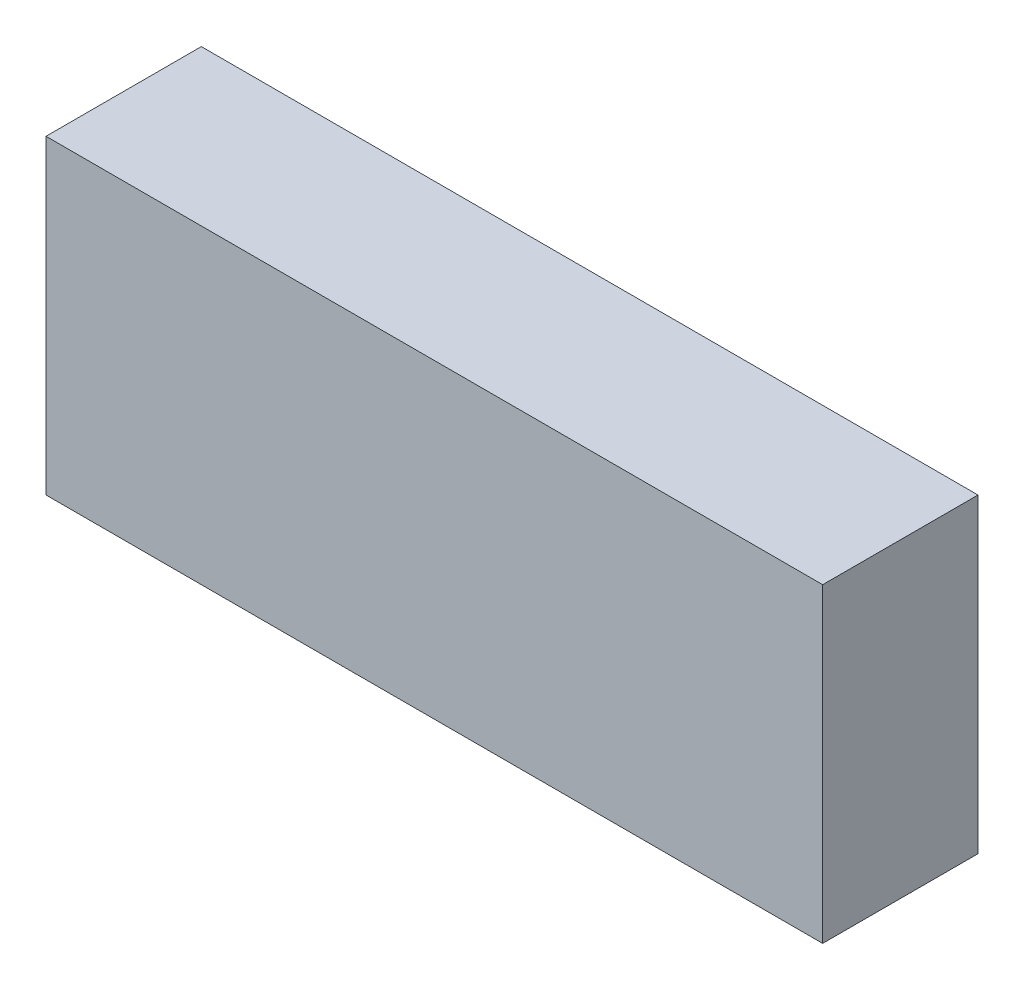
SolidWorks part; units mm, degrees
material "1023 碳钢板 (SS)"
ref_plane "Front Plane" through (0, 0, 0) normal (0, 0, 1) x (1, 0, 0)
ref_plane "Top Plane" through (0, 0, 0) normal (0, 1, 0) x (1, 0, 0)
ref_plane "Right Plane" through (0, 0, 0) normal (1, 0, 0) x (0, 0, -1)
sketch "Sketch1" plane through (0, 0, 0) normal (0, 0, 1) x (1, 0, 0)
  line L1 (-25, 10) -> (25, 10)
  line L2 (-25, 10) -> (-25, -10)
  line L3 (-25, -10) -> (25, -10)
  line L4 (25, 10) -> (25, -10)
  line L5 (-25, 10) -> (25, -10) construction
  line L6 (-25, -10) -> (25, 10) construction
  point P0 (0, 0)
  dimension "D1" = 50
  dimension "D2" = 20
extrude "Boss-Extrude1" add sketch "Sketch1" along normal blind 10
